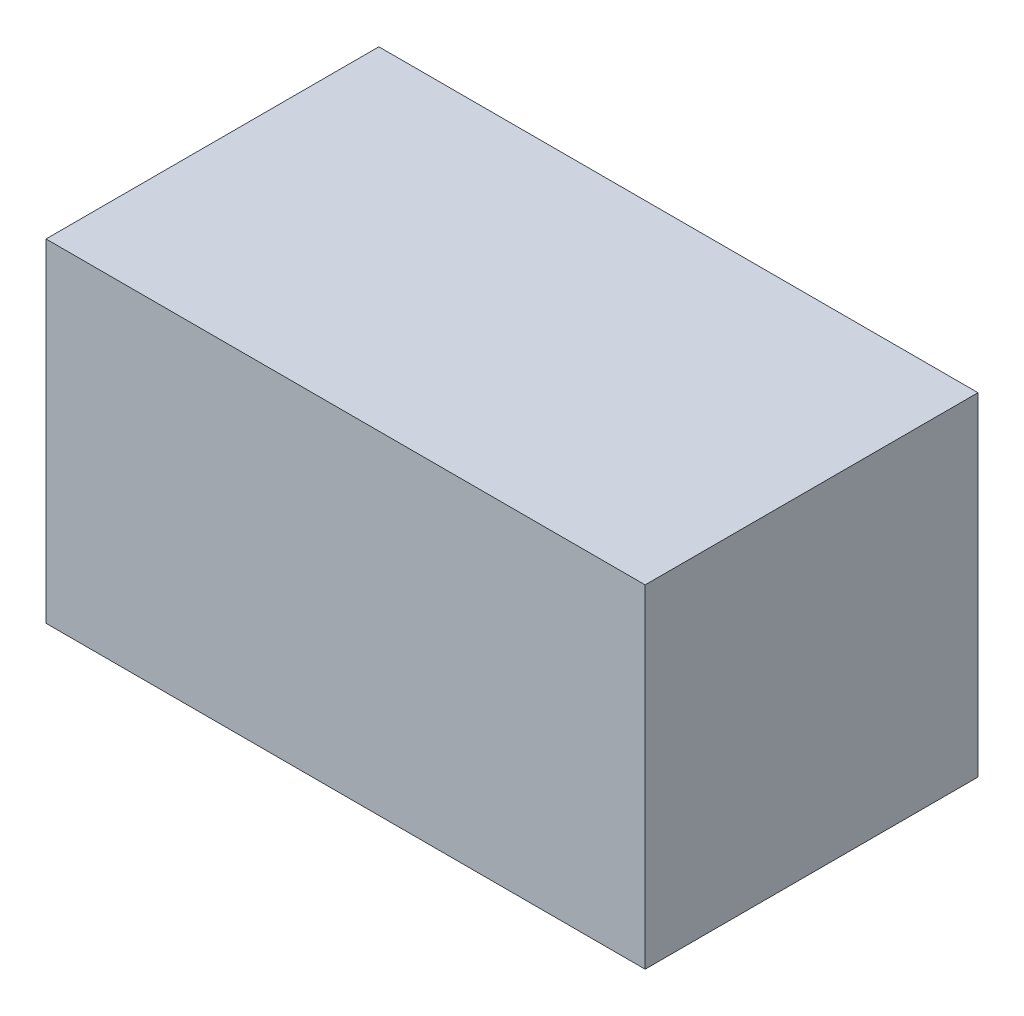
from build123d import *

# Parameters (mm, degrees)
SKETCH_1_W      = 18
SKETCH_1_H      = 10
EXTRUDE_1_DEPTH = 5


with BuildPart() as part:
    # 草图1 → 凸台-拉伸1 (new, symmetric)
    with BuildSketch(Plane.XY):
        Rectangle(SKETCH_1_W, SKETCH_1_H)
    extrude(amount=EXTRUDE_1_DEPTH, both=True)


solid = part.part
